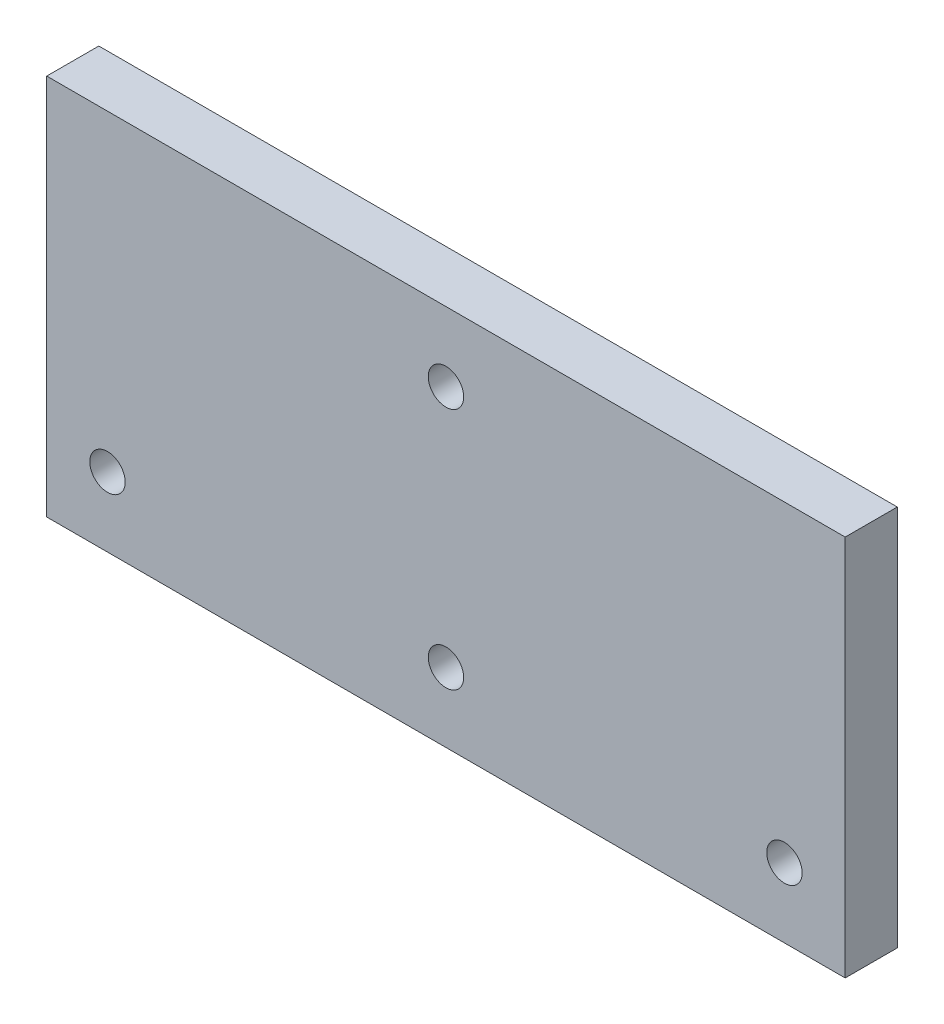
from build123d import *

# Parameters (mm, degrees)
SKETCH1_W              = 230
SKETCH1_H              = 110
BOSS_EXTRUDE1_DEPTH    = 15
M12_TAPPED_HOLE2_D     = 10.2
M12_TAPPED_HOLE2_DEPTH = 29.25
M12_TAPPED_HOLE2_TIP   = 3.064389157


with BuildPart() as part:
    # Sketch1 → Boss-Extrude1 (new body)
    with BuildSketch(Plane.XY):
        Rectangle(SKETCH1_W, SKETCH1_H)
    extrude(amount=BOSS_EXTRUDE1_DEPTH)

    # M12 Tapped Hole2
    with Locations(Plane.XY.offset(15)):
        with Locations((-97.5, -35), (97.5, -35), (0, 35), (0, -35)):
            Hole(M12_TAPPED_HOLE2_D / 2, depth=M12_TAPPED_HOLE2_DEPTH)
            with Locations((0, 0, -(M12_TAPPED_HOLE2_DEPTH + M12_TAPPED_HOLE2_TIP / 2))):  # 118° drill point
                Cone(0, M12_TAPPED_HOLE2_D / 2, M12_TAPPED_HOLE2_TIP, mode=Mode.SUBTRACT)


solid = part.part
